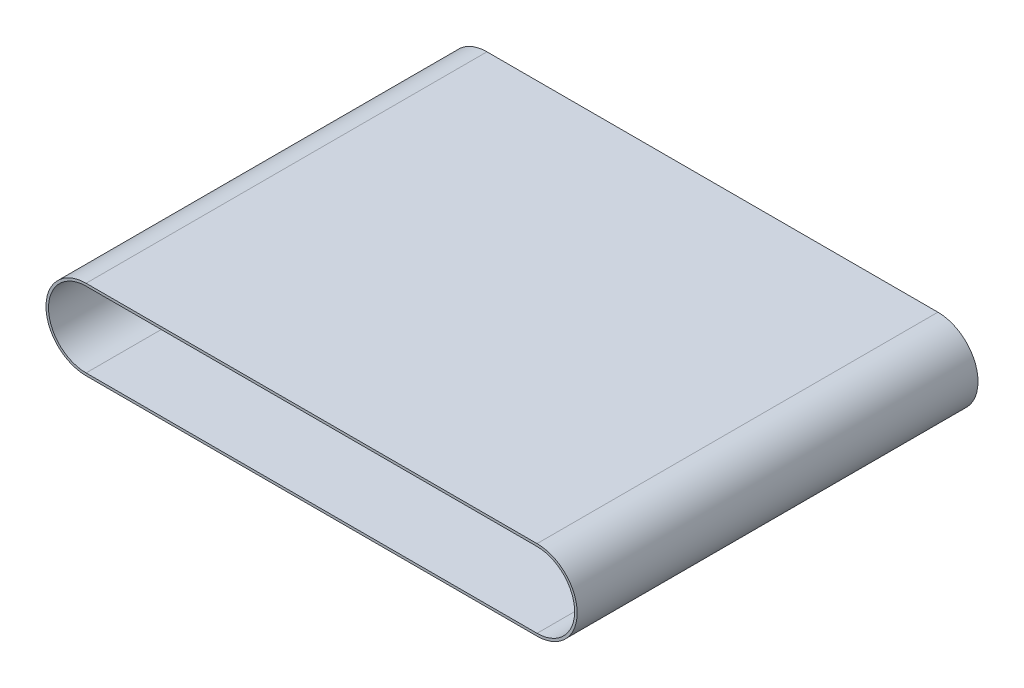
from build123d import *

# Parameters (mm, degrees)
EXTRUDE_1_DEPTH = 800


with BuildPart() as part:
    # 草图1 → 拉伸-薄壁1 (new body)
    with BuildSketch(Plane.XY):
        with BuildLine():
            Line((450, -74.939443754), (-450, -74.939443754))
            ThreePointArc((-450, -74.939443754), (-530, 5.060556246), (-450, 85.060556246))
            Line((-450, 85.060556246), (450, 85.060556246))
            ThreePointArc((450, 85.060556246), (530, 5.060556246), (450, -74.939443754))
        make_face()
        with BuildLine():
            Line((450, -69.939443754), (-450, -69.939443754))
            ThreePointArc((-450, -69.939443754), (-525, 5.060556246), (-450, 80.060556246))
            Line((-450, 80.060556246), (450, 80.060556246))
            ThreePointArc((450, 80.060556246), (525, 5.060556246), (450, -69.939443754))
        make_face(mode=Mode.SUBTRACT)
    extrude(amount=EXTRUDE_1_DEPTH)


solid = part.part
